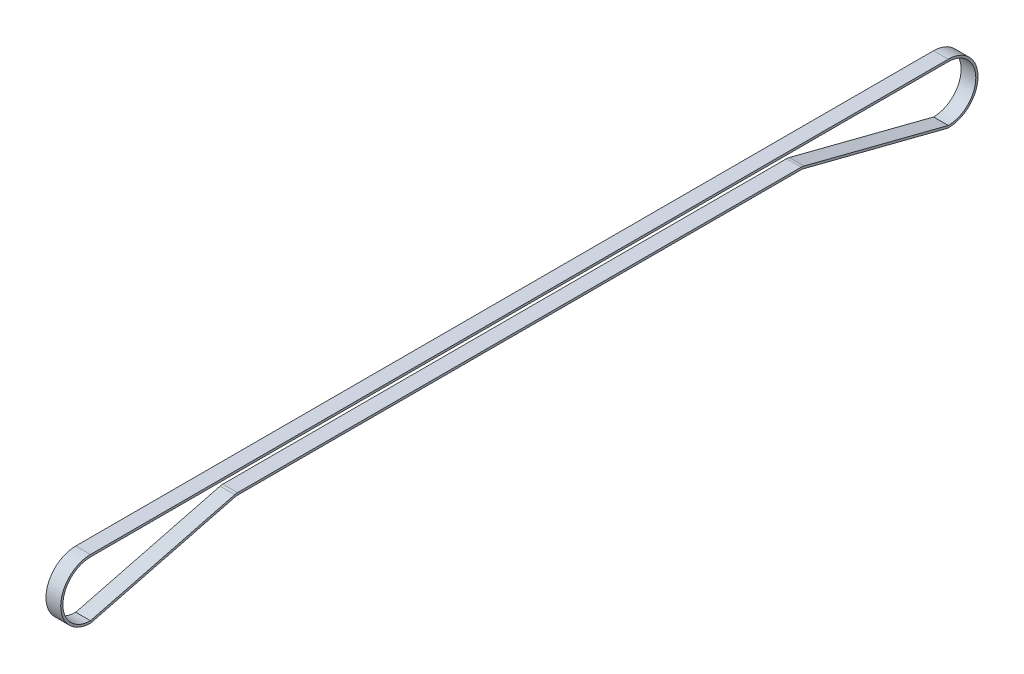
from build123d import *

# Parameters (mm, degrees)
EXTRUDE_1_DEPTH = 15


with BuildPart() as part:
    # 草图2 → 拉伸-薄壁1 (new, symmetric)
    with BuildSketch(Plane(origin=(0, 0, 0), x_dir=(0, 0, -1), z_dir=(1, 0, 0))):
        with BuildLine():
            Line((-295.400568077, 14.914130168), (-0.448465098, -60.793345886))
            ThreePointArc((-0.448465098, -60.793345886), (60.79458647, -0.224234074), (0, 60.795))
            Line((0, 60.795), (-1750, 60.795))
            ThreePointArc((-1750, 60.795), (-1810.79458647, -0.224234074), (-1749.551534902, -60.793345886))
            Line((-1749.551534902, -60.793345886), (-1454.599431923, 14.914130168))
            ThreePointArc((-1454.599431923, 14.914130168), (-1452.317983163, 15.349208075), (-1450, 15.495))
            Line((-1450, 15.495), (-300, 15.495))
            ThreePointArc((-300, 15.495), (-297.682016837, 15.349208075), (-295.400568077, 14.914130168))
        make_face()
        with BuildLine():
            Line((-294.281787339, 19.272837507), (0.125744515, -56.294859564))
            ThreePointArc((0.125744515, -56.294859564), (56.294964891, 0.062872297), (0, 56.295))
            Line((0, 56.295), (-1750, 56.295))
            ThreePointArc((-1750, 56.295), (-1806.294964891, 0.062872297), (-1750.125744515, -56.294859564))
            Line((-1750.125744515, -56.294859564), (-1455.718212661, 19.272837507))
            ThreePointArc((-1455.718212661, 19.272837507), (-1452.881816905, 19.813745174), (-1450, 19.995))
            Line((-1450, 19.995), (-300, 19.995))
            ThreePointArc((-300, 19.995), (-297.118183095, 19.813745174), (-294.281787339, 19.272837507))
        make_face(mode=Mode.SUBTRACT)
    extrude(amount=EXTRUDE_1_DEPTH, both=True)


solid = part.part
